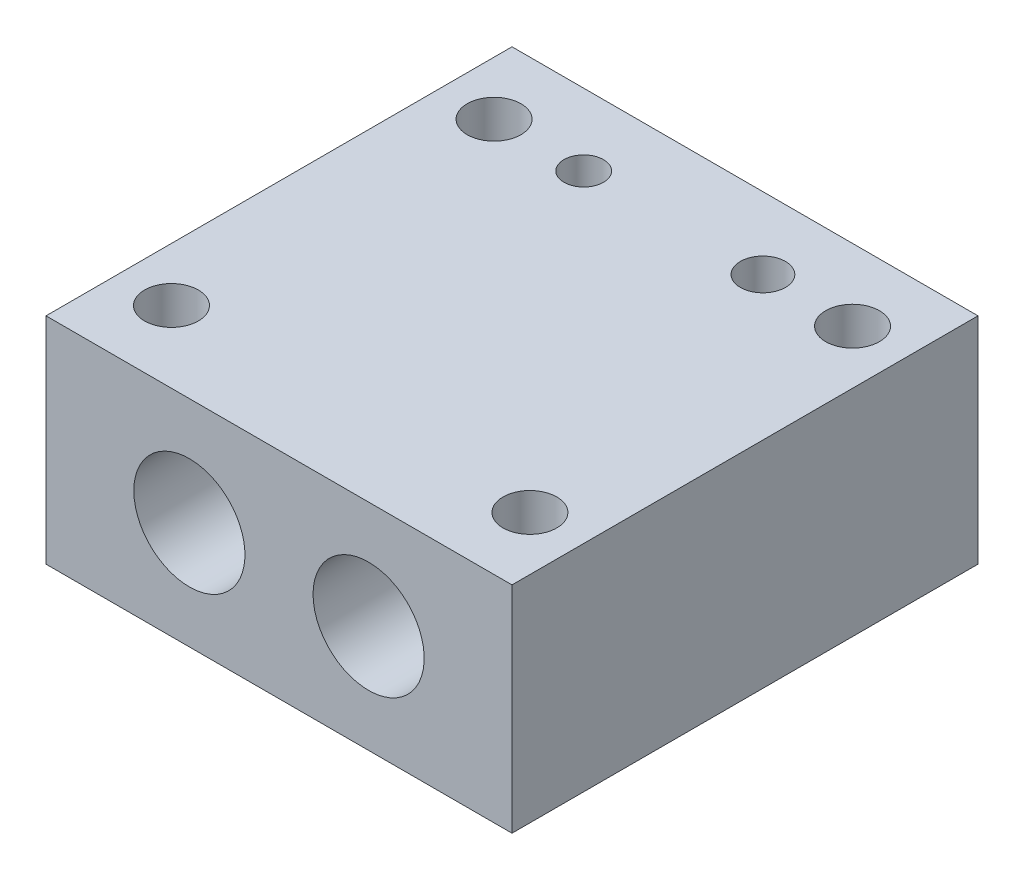
SolidWorks part; units mm, degrees
ref_plane "Front Plane" through (0, 0, 0) normal (0, 0, 1) x (1, 0, 0)
ref_plane "Top Plane" through (0, 0, 0) normal (0, 1, 0) x (1, 0, 0)
ref_plane "Right Plane" through (0, 0, 0) normal (1, 0, 0) x (0, 0, -1)
sketch "Sketch1" plane through (0, 0, 0) normal (0, 1, 0) x (1, 0, 0)
  line L1 (-65, -65) -> (65, -65)
  line L2 (-65, -65) -> (-65, 65)
  line L3 (-65, 65) -> (65, 65)
  line L4 (65, -65) -> (65, 65)
  line L5 (-65, -65) -> (65, 65) construction
  line L6 (-65, 65) -> (65, -65) construction
  point P0 (0, 0)
  dimension "D1" = 130
  dimension "D2" = 130
extrude "Boss-Extrude1" add sketch "Sketch1" along normal blind 60
sketch "Sketch2" plane through (0, 0, -65) normal (0, 0, -1) x (-1, 0, 0)
  line L0 (-65, 0) -> (65, 0) construction
  circle A0 centre (-25, 30) radius 15.5
  circle A1 centre (25, 30) radius 15.5
  dimension "D1" = 31
  dimension "D2" = 31
  dimension "D3" = 30
  dimension "D4" = 30
  dimension "D5" = 25
  dimension "D6" = 50
extrude "Cut-Extrude1" cut sketch "Sketch2" against normal blind 204
sketch "Sketch3" plane through (0, 60, 0) normal (0, 1, 0) x (1, 0, 0)
  line L1 (-50, -45) -> (50, -45) construction
  line L2 (-50, -45) -> (-50, 45) construction
  line L3 (-50, 45) -> (50, 45) construction
  line L4 (50, -45) -> (50, 45) construction
  line L5 (-50, -45) -> (50, 45) construction
  line L6 (-50, 45) -> (50, -45) construction
  circle A0 centre (-50, 45) radius 7.5
  circle A1 centre (50, 45) radius 7.5
  circle A2 centre (50, -45) radius 7.5
  circle A3 centre (-50, -45) radius 7.5
  point P0 (0, 0)
  dimension "D3" = 15
  dimension "D4" = 15
  dimension "D5" = 15
  dimension "D6" = 15
  dimension "D1" = 100
  dimension "D2" = 90
extrude "Cut-Extrude2" cut sketch "Sketch3" against normal blind 40
sketch "Sketch4" plane through (0, 20, 0) normal (0, 1, 0) x (1, 0, 0)
  circle A0 centre (50, 45) radius 4.1
  circle A1 centre (-50, 45) radius 4.1
  circle A2 centre (-50, -45) radius 4.1
  circle A3 centre (50, -45) radius 4.1
  dimension "D1" = 8.2
  dimension "D2" = 8.2
  dimension "D3" = 8.2
  dimension "D4" = 8.2
extrude "Cut-Extrude3" cut sketch "Sketch4" against normal blind 40
sketch "Sketch5" plane through (0, 60, 0) normal (0, 1, 0) x (1, 0, 0)
  line L3 (65, 65) -> (-65, 65) construction
  circle A0 centre (25, 45) radius 6.2943
  circle A2 centre (-25, 45) radius 5.5
  dimension "D3" = 11
  dimension "D4" = 25
  dimension "D5" = 20
  dimension "D1" = 25
  dimension "D2" = 20
extrude "Cut-Extrude4" cut sketch "Sketch5" against normal blind 104
